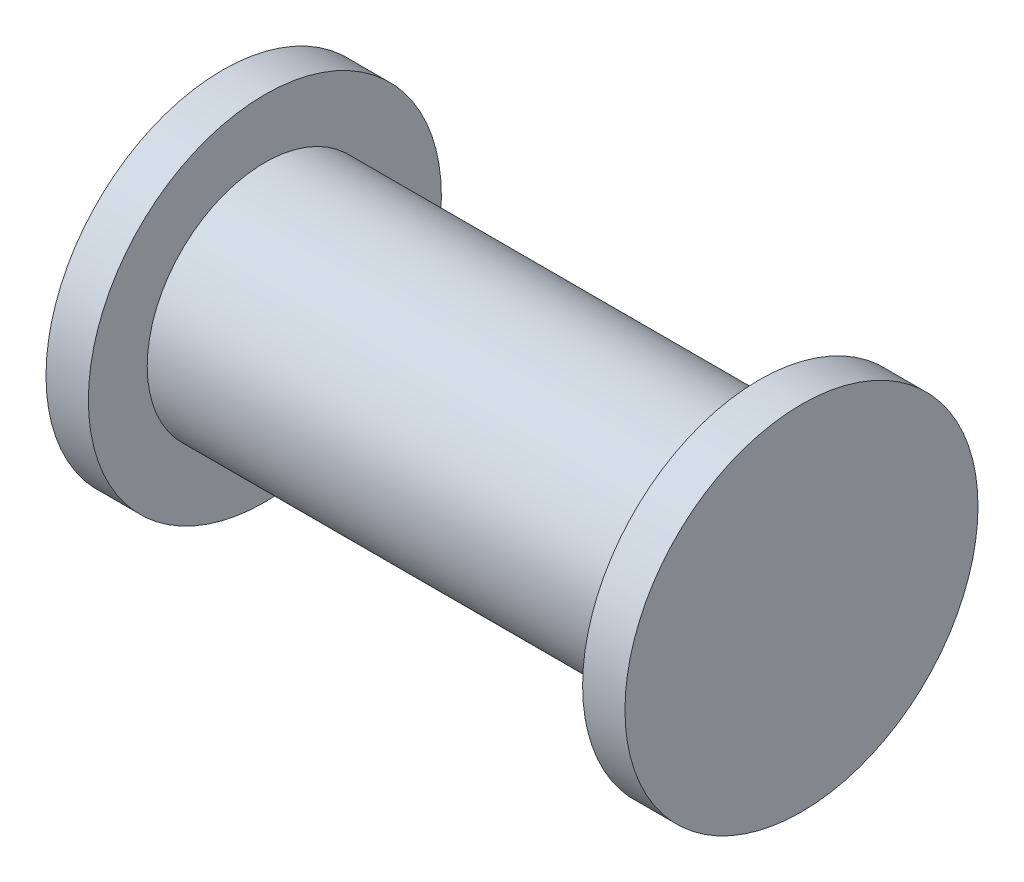
from build123d import *

# Parameters (mm, degrees)
SKETCH_1_4_R        = 75
BOSS_EXTRUDE1_DEPTH = 18
SKETCH_1_3_R        = 50
BOSS_EXTRUDE2_DEPTH = 210
BOSS_EXTRUDE3_START = -228
SKETCH_1_4_2_R      = 75
BOSS_EXTRUDE3_DEPTH = 18


with BuildPart() as part:
    # Sketch 1_4 → Boss-Extrude1 (new body)
    with BuildSketch(Plane(origin=(0, 0, 0), x_dir=(0, 0, -1), z_dir=(1, 0, 0))):
        Circle(SKETCH_1_4_R)
    extrude(amount=BOSS_EXTRUDE1_DEPTH)

    # 草图1<3> → Boss-Extrude2 (add)
    with BuildSketch(Plane(origin=(0, 0, 0), x_dir=(0, 0, -1), z_dir=(1, 0, 0))):
        Circle(SKETCH_1_3_R)
    extrude(amount=-BOSS_EXTRUDE2_DEPTH)

    # Sketch 1_4 2 → Boss-Extrude3 (add)
    with BuildSketch(Plane(origin=(0, 0, 0), x_dir=(0, 0, -1), z_dir=(1, 0, 0)).offset(BOSS_EXTRUDE3_START)):
        Circle(SKETCH_1_4_2_R)
    extrude(amount=BOSS_EXTRUDE3_DEPTH)


solid = part.part
